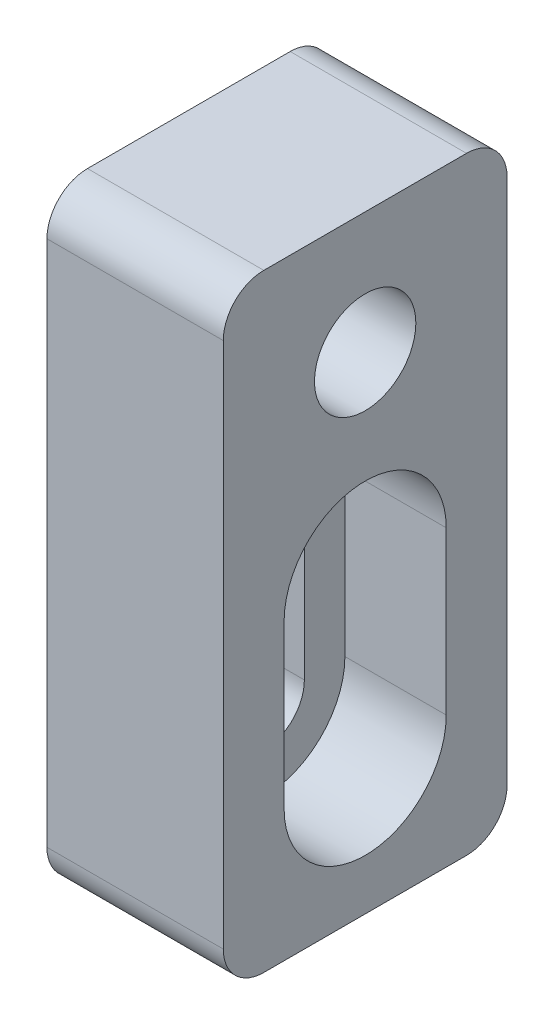
from build123d import *

# Parameters (mm, degrees)
SKETCH_1_W          = 8.7
SKETCH_1_H          = 30
EXTRUDE_1_DEPTH     = 14
HOLE_WIZARD_M6_1_D  = 5
CUT_EXTRUDE_1_DEPTH = 23.286543025
CUT_EXTRUDE_2_DEPTH = 5
FILLET_1_R          = 2


with BuildPart() as part:
    # 草图1 → 凸台-拉伸1 (new body)
    with BuildSketch(Plane.XY):
        Rectangle(SKETCH_1_W, SKETCH_1_H)
    extrude(amount=EXTRUDE_1_DEPTH)

    # M6 螺纹孔1 (through all)
    with Locations(Plane(origin=(4.35, 0, 0), x_dir=(0, 0, -1), z_dir=(1, 0, 0))):
        with Locations((-7, 9)):
            Hole(HOLE_WIZARD_M6_1_D / 2)

    # 草图4 → 切除-拉伸1 (cut, through all)
    with BuildSketch(Plane(origin=(4.35, 0, 0), x_dir=(0, 0, -1), z_dir=(1, 0, 0))):
        with BuildLine():
            Line((-9, -8.5), (-9, -0.5))
            ThreePointArc((-9, -0.5), (-7, 1.5), (-5, -0.5))
            Line((-5, -0.5), (-5, -8.5))
            ThreePointArc((-5, -8.5), (-7, -10.5), (-9, -8.5))
        make_face()
    extrude(amount=-CUT_EXTRUDE_1_DEPTH, mode=Mode.SUBTRACT)

    # 草图5 → 切除-拉伸2 (cut)
    with BuildSketch(Plane(origin=(4.35, 0, 0), x_dir=(0, 0, -1), z_dir=(1, 0, 0))):
        with BuildLine():
            Line((-3, -0.5), (-3, -8.5))
            ThreePointArc((-3, -8.5), (-7, -12.5), (-11, -8.5))
            Line((-11, -8.5), (-11, -0.5))
            ThreePointArc((-11, -0.5), (-7, 3.5), (-3, -0.5))
        make_face()
    extrude(amount=-CUT_EXTRUDE_2_DEPTH, mode=Mode.SUBTRACT)

    # 圆角1
    fillet_1_edges = [part.edges().sort_by_distance(p)[0] for p in [
        (0, -15, 14),
        (0, -15, 0),
        (0, 15, 0),
        (0, 15, 14),
    ]]
    fillet(fillet_1_edges, radius=FILLET_1_R)


solid = part.part
